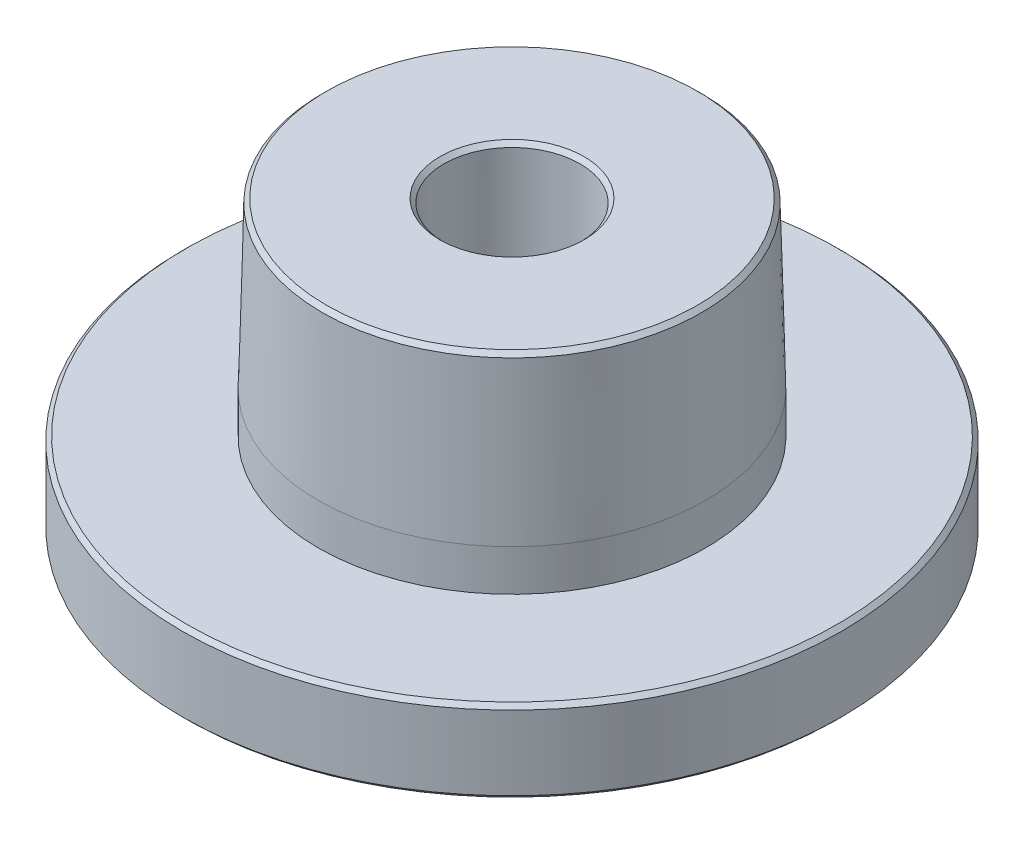
SolidWorks part; units mm, degrees
ref_plane "Front Plane" through (0, 0, 0) normal (0, 0, 1) x (1, 0, 0)
ref_plane "Top Plane" through (0, 0, 0) normal (0, 1, 0) x (1, 0, 0)
ref_plane "Right Plane" through (0, 0, 0) normal (1, 0, 0) x (0, 0, -1)
sketch "Sketch1" plane through (0, 0, 0) normal (0, 0, 1) x (1, 0, 0)
  line L0 (8.25, 35) -> (23, 35)
  line L1 (23, 35) -> (23.5, 15)
  line L2 (23.5, 15) -> (23.5, 10)
  line L3 (23.5, 10) -> (40, 10)
  line L4 (40, 10) -> (40, 0)
  line L5 (40, 0) -> (8.25, 0)
  line L6 (0, 0) -> (0, 36.7634) construction
  line L7 (8.25, 35) -> (8.25, 0)
  dimension "D1" = 8.25
  dimension "D2" = 40
  dimension "D3" = 23.5
  dimension "D4" = 23
  dimension "D5" = 35
  dimension "D6" = 10
  dimension "D7" = 5
revolve "Revolve1" add sketch "Sketch1" angle 360 about L6
chamfer "Chamfer1" distance 0.5 angle 45 5 edges at (0, 0, -40) (0, 10, -40) (0, 35, -23) (0, 35, -8.25) (0, 0, -8.25)
